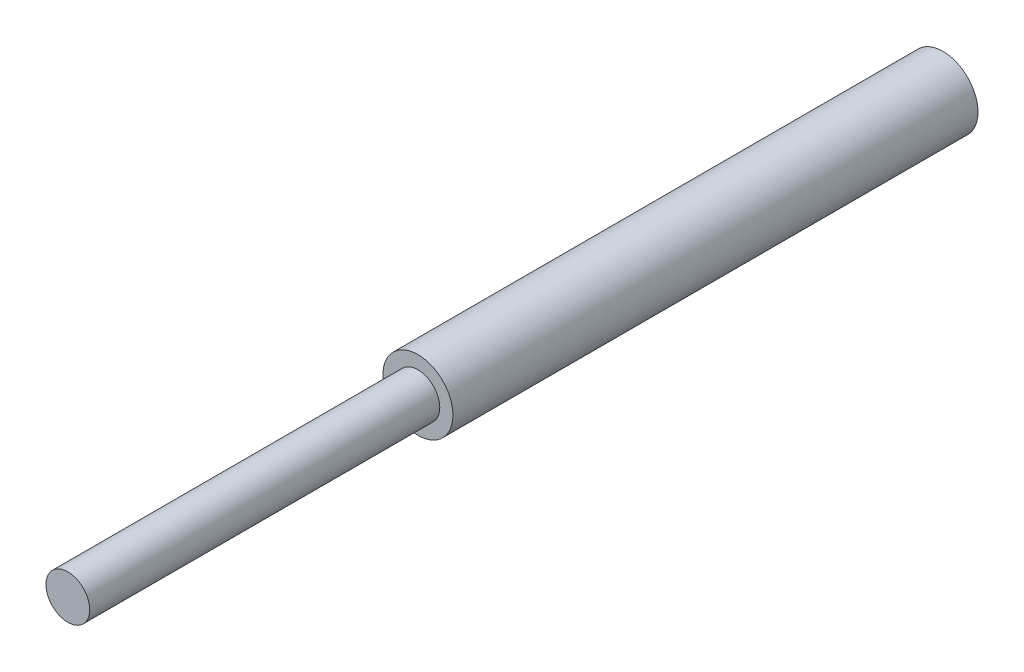
SolidWorks part; units mm, degrees
ref_plane "前视基准面" through (0, 0, 0) normal (0, 0, 1) x (1, 0, 0)
ref_plane "上视基准面" through (0, 0, 0) normal (0, 1, 0) x (1, 0, 0)
ref_plane "右视基准面" through (0, 0, 0) normal (1, 0, 0) x (0, 0, -1)
sketch "草图1" plane through (0, 0, 0) normal (0, 0, 1) x (1, 0, 0)
  circle A0 centre (0, 0) radius 4
  dimension "D1" = 8
extrude "凸台-拉伸1" add sketch "草图1" along normal blind 100
sketch "草图2" plane through (0, 0, 100) normal (0, 0, 1) x (1, 0, 0)
  circle A0 centre (0, 0) radius 2.5
  circle A2 centre (0, 0) radius 4
  dimension "D1" = 5
extrude "切除-拉伸1" cut sketch "草图2" against normal blind 40
